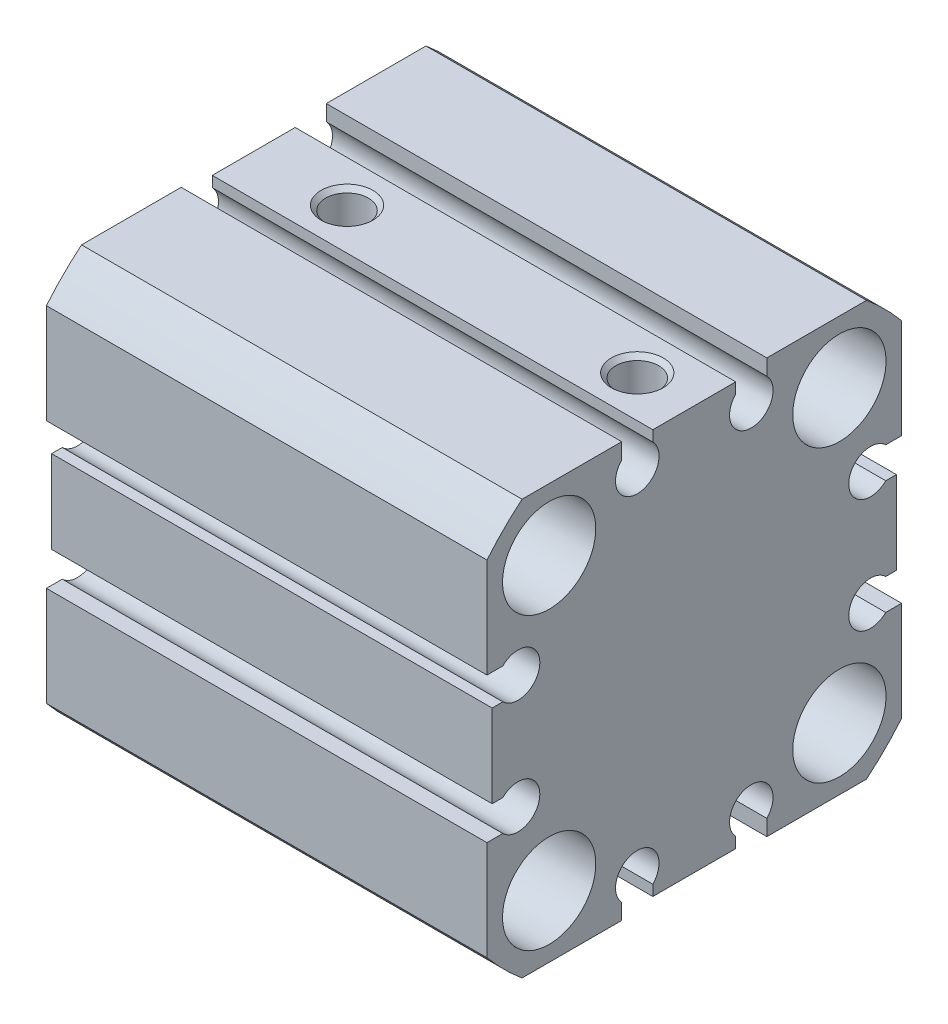
from build123d import *

# Parameters (mm, degrees)
BOSS_EXTRUDE1_DEPTH  = 42.5
LPATTERN1_COUNT      = 2
LPATTERN1_PITCH      = 28
LPATTERN1_COUNT_DIR2 = 2
LPATTERN1_PITCH_DIR2 = 28
HOLE1_D              = 4.134
HOLE1_DEPTH          = 5
HOLE1_CSINK_D        = 5
HOLE1_CSINK_ANGLE    = 90
HOLE1_TIP            = 1.193383006
HOLE2_D              = 4.134
HOLE2_DEPTH          = 5
HOLE2_CSINK_D        = 5
HOLE2_CSINK_ANGLE    = 90
HOLE2_TIP            = 1.193383006


with BuildPart() as part:
    # Sketch1 → Boss-Extrude1 (new body)
    with BuildSketch(Plane(origin=(0, 0, 0), x_dir=(0, 0, -1), z_dir=(1, 0, 0))):
        with BuildLine():
            Line((-16.613247726, -20), (-7, -20))
            Line((-7, -20), (-7, -18.469693846))
            ThreePointArc((-7, -18.469693846), (-5.5, -14.9), (-4, -18.469693846))
            Line((-4, -18.469693846), (-4, -19.5))
            Line((-4, -19.5), (4, -19.5))
            Line((4, -19.5), (4, -18.469693846))
            ThreePointArc((4, -18.469693846), (5.5, -14.9), (7, -18.469693846))
            Line((7, -18.469693846), (7, -20))
            Line((7, -20), (16.613247726, -20))
            ThreePointArc((16.613247726, -20), (18.384776311, -18.384776311), (20, -16.613247726))
            Line((20, -16.613247726), (20, -7))
            Line((20, -7), (18.469693846, -7))
            ThreePointArc((18.469693846, -7), (14.9, -5.5), (18.469693846, -4))
            Line((18.469693846, -4), (19.5, -4))
            Line((19.5, -4), (19.5, 4))
            Line((19.5, 4), (18.469693846, 4))
            ThreePointArc((18.469693846, 4), (14.9, 5.5), (18.469693846, 7))
            Line((18.469693846, 7), (20, 7))
            Line((20, 7), (20, 16.613247726))
            ThreePointArc((20, 16.613247726), (18.384776311, 18.384776311), (16.613247726, 20))
            Line((16.613247726, 20), (7, 20))
            Line((7, 20), (7, 18.469693846))
            ThreePointArc((7, 18.469693846), (5.5, 14.9), (4, 18.469693846))
            Line((4, 18.469693846), (4, 19.5))
            Line((4, 19.5), (-4, 19.5))
            Line((-4, 19.5), (-4, 18.469693846))
            ThreePointArc((-4, 18.469693846), (-5.5, 14.9), (-7, 18.469693846))
            Line((-7, 18.469693846), (-7, 20))
            Line((-7, 20), (-16.613247726, 20))
            ThreePointArc((-16.613247726, 20), (-18.384776311, 18.384776311), (-20, 16.613247726))
            Line((-20, 16.613247726), (-20, 7))
            Line((-20, 7), (-18.469693846, 7))
            ThreePointArc((-18.469693846, 7), (-14.9, 5.5), (-18.469693846, 4))
            Line((-18.469693846, 4), (-19.5, 4))
            Line((-19.5, 4), (-19.5, -4))
            Line((-19.5, -4), (-18.469693846, -4))
            ThreePointArc((-18.469693846, -4), (-14.9, -5.5), (-18.469693846, -7))
            Line((-18.469693846, -7), (-20, -7))
            Line((-20, -7), (-20, -16.613247726))
            ThreePointArc((-20, -16.613247726), (-18.384776311, -18.384776311), (-16.613247726, -20))
        make_face()
    extrude(amount=BOSS_EXTRUDE1_DEPTH)

    # Sketch2 → Cut-Revolve1 (revolve, cut)
    with BuildSketch(Plane.XY.offset(14), mode=Mode.PRIVATE) as cut_revolve1_sk:
        Polygon((0, 14), (0, 18.5), (7, 18.5), (7, 17), (7.5415, 16.4585), (17, 16.4585), (17.13943009, 16.7), (25.36056991, 16.7), (25.5, 16.4585), (34.9585, 16.4585), (35.5, 17), (35.5, 18.5), (42.5, 18.5), (42.5, 14), align=None)
    cut_revolve1 = revolve(cut_revolve1_sk.sketch.rotate(Axis((42.5, 14, 14), (-1, 0, 0)), 270), axis=Axis((42.5, 14, 14), (-1, 0, 0)), mode=Mode.SUBTRACT)

    # LPattern1: Cut-Revolve1 2 × 2
    with Locations(*[(0, -j * LPATTERN1_PITCH_DIR2, -i * LPATTERN1_PITCH) for i in range(LPATTERN1_COUNT) for j in range(LPATTERN1_COUNT_DIR2) if (i, j) != (0, 0)]):
        add(cut_revolve1, mode=Mode.SUBTRACT)

    # Sketch4 → Cut-Revolve2 (revolve, cut)
    with BuildSketch(Plane.XY, mode=Mode.PRIVATE) as cut_revolve2_sk:
        Polygon((0, 0), (0, 6), (16.25, 6), (16.25, 12.5), (31.25, 12.5), (31.25, 0), align=None)
    revolve(cut_revolve2_sk.sketch.rotate(Axis((31.25, 0, 0), (-1, 0, 0)), 270), axis=Axis((31.25, 0, 0), (-1, 0, 0)), mode=Mode.SUBTRACT)

    # Hole1
    with Locations(Plane(origin=(0, 19.5, 0), x_dir=(-1, 0, 0), z_dir=(0, 1, 0))):
        with Locations((-9, 0)):
            CounterSinkHole(HOLE1_D / 2, HOLE1_CSINK_D / 2, depth=HOLE1_DEPTH, counter_sink_angle=HOLE1_CSINK_ANGLE)
            with Locations((0, 0, -(HOLE1_DEPTH + HOLE1_TIP / 2))):  # 120° drill point
                Cone(0, HOLE1_D / 2, HOLE1_TIP, mode=Mode.SUBTRACT)

    # Hole2
    with Locations(Plane(origin=(0, 19.5, 0), x_dir=(-1, 0, 0), z_dir=(0, 1, 0))):
        with Locations((-37, 0)):
            CounterSinkHole(HOLE2_D / 2, HOLE2_CSINK_D / 2, depth=HOLE2_DEPTH, counter_sink_angle=HOLE2_CSINK_ANGLE)
            with Locations((0, 0, -(HOLE2_DEPTH + HOLE2_TIP / 2))):  # 120° drill point
                Cone(0, HOLE2_D / 2, HOLE2_TIP, mode=Mode.SUBTRACT)


solid = part.part
